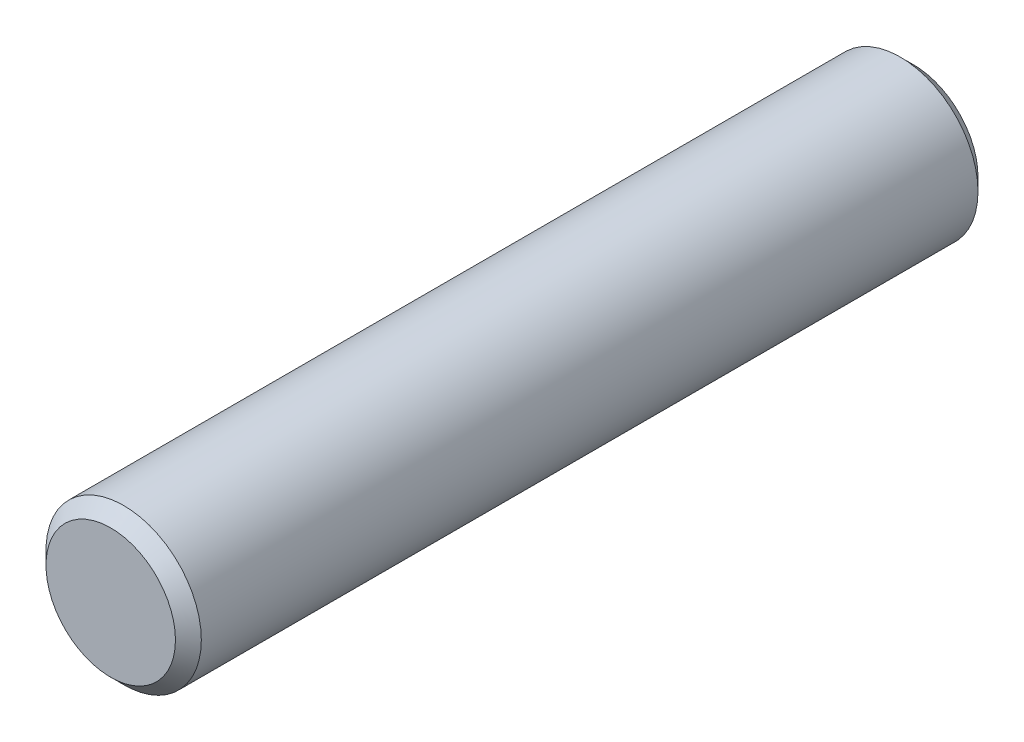
SolidWorks part; units mm, degrees
ref_plane "Front Plane" through (0, 0, 0) normal (0, 0, 1) x (1, 0, 0)
ref_plane "Top Plane" through (0, 0, 0) normal (0, 1, 0) x (1, 0, 0)
ref_plane "Right Plane" through (0, 0, 0) normal (1, 0, 0) x (0, 0, -1)
sketch "Sketch1" plane through (0, 0, 0) normal (0, 0, 1) x (1, 0, 0)
  circle A0 centre (0, 0) radius 0.6
  dimension "D1" = 1.2
extrude "Boss-Extrude1" add sketch "Sketch1" along normal mid plane 6.2
chamfer "Chamfer1" distance 0.1 angle 45 2 edges at (0.6, 0, -3.1) (0.6, 0, 3.1)
